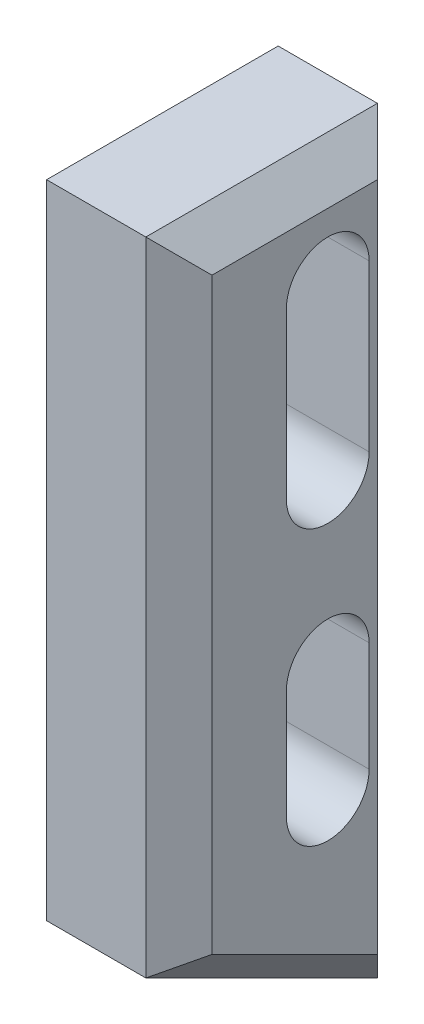
from build123d import *

# Parameters (mm, degrees)
BOSS_EXTRUDE1_DEPTH = 20
CHAMFER1_SIZE       = 10


with BuildPart() as part:
    # Sketch1 → Boss-Extrude1 (new, symmetric)
    with BuildSketch(Plane(origin=(0, 0, 0), x_dir=(0, 0, -1), z_dir=(1, 0, 0))):
        Polygon((0, 0), (70, -35), (70, 194), (0, 194), align=None)
        with BuildLine():
            Line((32.5, 114), (32.5, 164))
            ThreePointArc((32.5, 164), (45, 176.5), (57.5, 164))
            Line((57.5, 164), (57.5, 114))
            ThreePointArc((57.5, 114), (45, 101.5), (32.5, 114))
        make_face(mode=Mode.SUBTRACT)
        with BuildLine():
            Line((32.5, 30.910324642), (32.5, 64))
            ThreePointArc((32.5, 64), (45, 76.5), (57.5, 64))
            Line((57.5, 64), (57.5, 30.910324642))
            ThreePointArc((57.5, 30.910324642), (45, 18.410324642), (32.5, 30.910324642))
        make_face(mode=Mode.SUBTRACT)
    extrude(amount=BOSS_EXTRUDE1_DEPTH, both=True)

    # Chamfer1
    chamfer1_edges = [part.edges().sort_by_distance(p)[0] for p in [
        (20, 79.5, -70),
        (20, 194, -35),
        (20, 97, 0),
        (20, -17.5, -35),
    ]]
    chamfer(chamfer1_edges, length=CHAMFER1_SIZE)


solid = part.part
